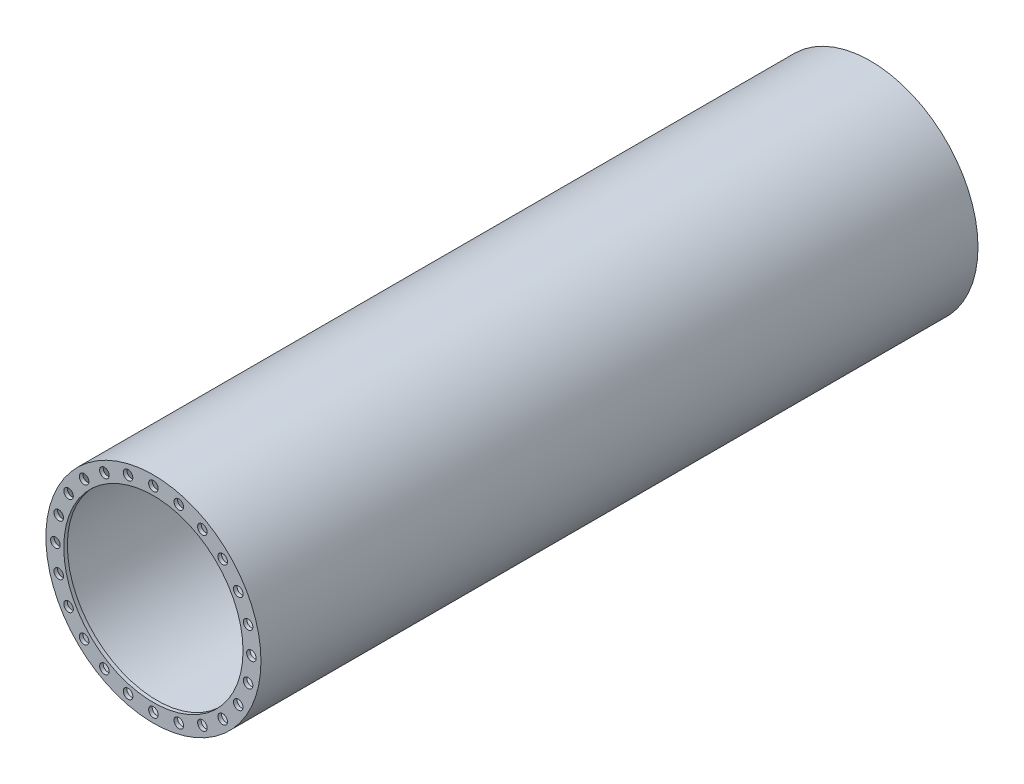
from build123d import *

# Parameters (mm, degrees)
SKETCH_1_R          = 450
SKETCH_1_R_2        = 442
EXTRUDE_1_DEPTH     = 1500
SKETCH_2_R          = 450
SKETCH_2_R_2        = 375
EXTRUDE_3_DEPTH     = 15
SKETCH_3_R          = 20
CUT_EXTRUDE_1_DEPTH = 3067.757245039


with BuildPart() as part:
    # 草图1 → 凸台-拉伸1 (new, symmetric)
    with BuildSketch(Plane.XY):
        Circle(SKETCH_1_R)
        Circle(SKETCH_1_R_2, mode=Mode.SUBTRACT)
    extrude(amount=EXTRUDE_1_DEPTH, both=True)

    # 草图2 → 凸台-拉伸3 (add)
    with BuildSketch(Plane.XY.offset(1500)):
        Circle(SKETCH_2_R)
        Circle(SKETCH_2_R_2, mode=Mode.SUBTRACT)
    extrude_3 = extrude(amount=-EXTRUDE_3_DEPTH)

    # 镜向1: 凸台-拉伸3 across plane
    add(extrude_3.mirror(Plane.XY))

    # 草图3 → 切除-拉伸1 (cut, through all)
    with BuildSketch(Plane.XY.offset(1500)):
        with Locations((0, 410)):
            Circle(SKETCH_3_R)
        with Locations((106.115808492, 396.029588779)):
            Circle(SKETCH_3_R)
        with Locations((205, 355.070415552)):
            Circle(SKETCH_3_R)
        with Locations((289.913780286, 289.913780286)):
            Circle(SKETCH_3_R)
        with Locations((355.070415552, 205)):
            Circle(SKETCH_3_R)
        with Locations((396.029588779, 106.115808492)):
            Circle(SKETCH_3_R)
        with Locations((410, 0)):
            Circle(SKETCH_3_R)
        with Locations((396.029588779, -106.115808492)):
            Circle(SKETCH_3_R)
        with Locations((355.070415552, -205)):
            Circle(SKETCH_3_R)
        with Locations((289.913780286, -289.913780286)):
            Circle(SKETCH_3_R)
        with Locations((205, -355.070415552)):
            Circle(SKETCH_3_R)
        with Locations((106.115808492, -396.029588779)):
            Circle(SKETCH_3_R)
        with Locations((0, -410)):
            Circle(SKETCH_3_R)
        with Locations((-106.115808492, -396.029588779)):
            Circle(SKETCH_3_R)
        with Locations((-205, -355.070415552)):
            Circle(SKETCH_3_R)
        with Locations((-289.913780286, -289.913780286)):
            Circle(SKETCH_3_R)
        with Locations((-355.070415552, -205)):
            Circle(SKETCH_3_R)
        with Locations((-396.029588779, -106.115808492)):
            Circle(SKETCH_3_R)
        with Locations((-410, 0)):
            Circle(SKETCH_3_R)
        with Locations((-396.029588779, 106.115808492)):
            Circle(SKETCH_3_R)
        with Locations((-355.070415552, 205)):
            Circle(SKETCH_3_R)
        with Locations((-289.913780286, 289.913780286)):
            Circle(SKETCH_3_R)
        with Locations((-205, 355.070415552)):
            Circle(SKETCH_3_R)
        with Locations((-106.115808492, 396.029588779)):
            Circle(SKETCH_3_R)
    extrude(amount=-CUT_EXTRUDE_1_DEPTH, mode=Mode.SUBTRACT)


solid = part.part
